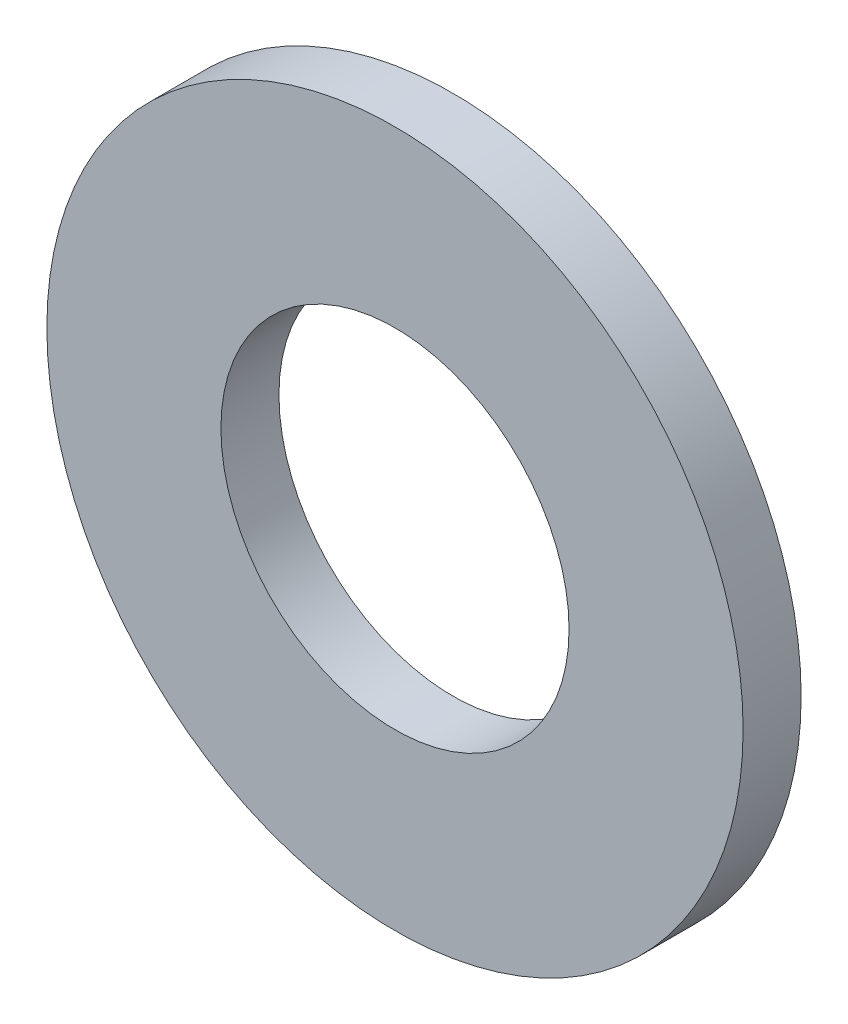
from build123d import *

# Parameters (mm, degrees)
SKETCH1_R           = 24
SKETCH1_R_2         = 12
BOSS_EXTRUDE1_DEPTH = 4


with BuildPart() as part:
    # Sketch1 → Boss-Extrude1 (new body)
    with BuildSketch(Plane.XY):
        Circle(SKETCH1_R)
        Circle(SKETCH1_R_2, mode=Mode.SUBTRACT)
    extrude(amount=BOSS_EXTRUDE1_DEPTH)


solid = part.part
